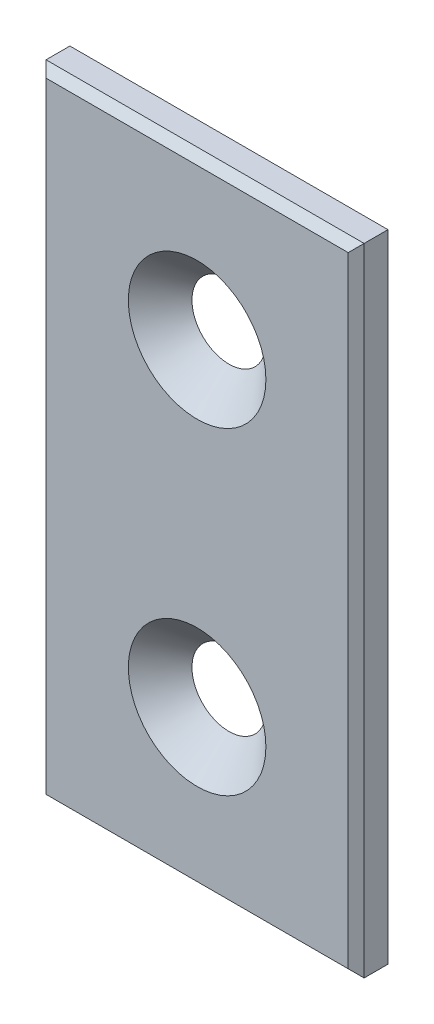
SolidWorks part; units mm, degrees
material "6061 合金"
ref_plane "前视基准面" through (0, 0, 0) normal (0, 0, 1) x (1, 0, 0)
ref_plane "上视基准面" through (0, 0, 0) normal (0, 1, 0) x (1, 0, 0)
ref_plane "右视基准面" through (0, 0, 0) normal (1, 0, 0) x (0, 0, -1)
sketch "草图1" plane through (0, 0, 0) normal (0, 0, 1) x (1, 0, 0)
  line L1 (-20, 40) -> (20, 40)
  line L2 (-20, 40) -> (-20, -40)
  line L3 (-20, -40) -> (20, -40)
  line L4 (20, 40) -> (20, -40)
  line L5 (-20, 40) -> (20, -40) construction
  line L6 (-20, -40) -> (20, 40) construction
  point P0 (0, 0)
  dimension "D1" = 40
  dimension "D2" = 80
extrude "凸台-拉伸1" add sketch "草图1" along normal mid plane 4
hole_wizard "打孔尺寸(%根据十字)槽沉头木螺钉的类型1" positions "3D草图1" profile "草图2" countersink size "M8" standard "GB"
sketch3d "3D草图1"
  line L0 (-20, -40, 2) -> (20, -40, 2) construction
  line L1 (-20, 40, 2) -> (-20, -40, 2) construction
  point P0 (0, 20, 2)
  point P2 (0, -20, 2)
  dimension "D1" = 40
  dimension "D2" = 20
  dimension "D3" = 20
  dimension "D4" = 20
sketch "草图2" plane through (0, 20, 2) normal (1, 0, 0) x (0, -1, 0)
  line L0 (0, 0) -> (0, 12.7039)
  line L1 (0, 12.7039) -> (4.5, 10)
  line L2 (4.5, 10) -> (4.5, 4.15)
  line L3 (4.5, 4.15) -> (8.65, 0)
  line L5 (8.65, 0) -> (0, 0)
  line L6 (-4.5, 4.15) -> (-8.65, 0) construction
  line L10 (0, 12.7039) -> (-4.5, 10) construction
  line L11 (0, -6.35) -> (0, 107.95) construction
  dimension "孔直径" = 9
  dimension "孔深度" = 10
  dimension "近端锥形沉头孔直径" = 17.3
  dimension "近端锥形沉头孔角度" = 90
  dimension "导头角度" = 118
chamfer "倒角1" distance 1 angle 45 4 edges at (0, -40, 2) (-20, 0, 2) (0, 40, 2) (20, 0, 2)
